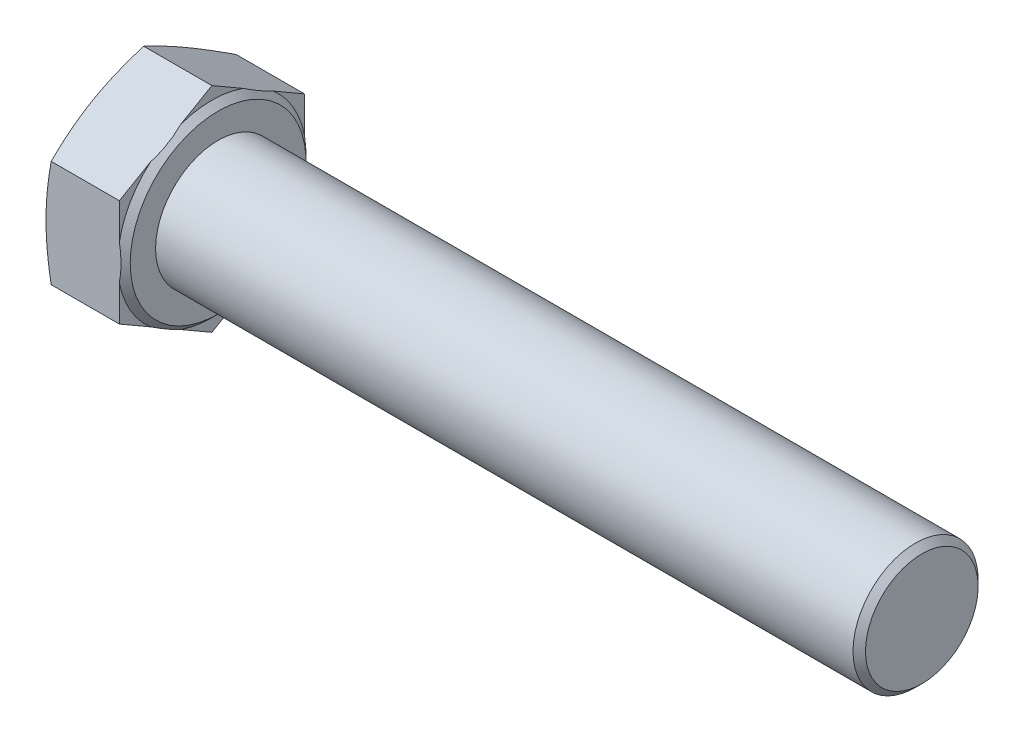
from build123d import *

# Parameters (mm, degrees)
BASEHEAD_DEPTH = 10.18
SKETCH5_R      = 8
BASEBODY_DEPTH = 90
CHAMFER1_SIZE  = 0.8


with BuildPart() as part:
    # Sketch2 → BaseHead (new body)
    with BuildSketch(Plane(origin=(0, 0, 0), x_dir=(0, 0, -1), z_dir=(1, 0, 0))):
        Polygon((11.835, -6.832940436), (11.835, 6.832940436), (0, 13.665880872), (-11.835, 6.832940436), (-11.835, -6.832940436), (0, -13.665880872), align=None)
    extrude(amount=BASEHEAD_DEPTH)

    # Sketch3 → BearingFace (revolve, cut)
    with BuildSketch(Plane.XY, mode=Mode.PRIVATE) as bearingface_sk:
        Polygon((10.18, 13.665880872), (10.18, 11.245), (9.38, 12.045), (9.38, 13.665880872), align=None)
    revolve(bearingface_sk.sketch.rotate(Axis((-0.957090588, 0, 0), (1, 0, 0)), 90), axis=Axis((-0.957090588, 0, 0), (1, 0, 0)), mode=Mode.SUBTRACT)

    # Sketch4 → Head chamfer (revolve, cut)
    with BuildSketch(Plane.XY):
        Polygon((0, 13.665880872), (0.66638614, 13.665880872), (0, 11.835), align=None)
    revolve(axis=Axis((-0.493528746, 0, 0), (1, 0, 0)), mode=Mode.SUBTRACT)

    # Sketch5 → BaseBody (add)
    with BuildSketch(Plane(origin=(10.18, 0, 0), x_dir=(0, 0, -1), z_dir=(1, 0, 0))):
        with Locations(Location((0, 0, 0), (0, 0, 180))):
            Circle(SKETCH5_R)
    extrude(amount=BASEBODY_DEPTH)

    # Chamfer1
    chamfer1_edges = [part.edges().sort_by_distance(p)[0] for p in [
        (100.18, 0, -8),
    ]]
    chamfer(chamfer1_edges, length=CHAMFER1_SIZE)


solid = part.part
